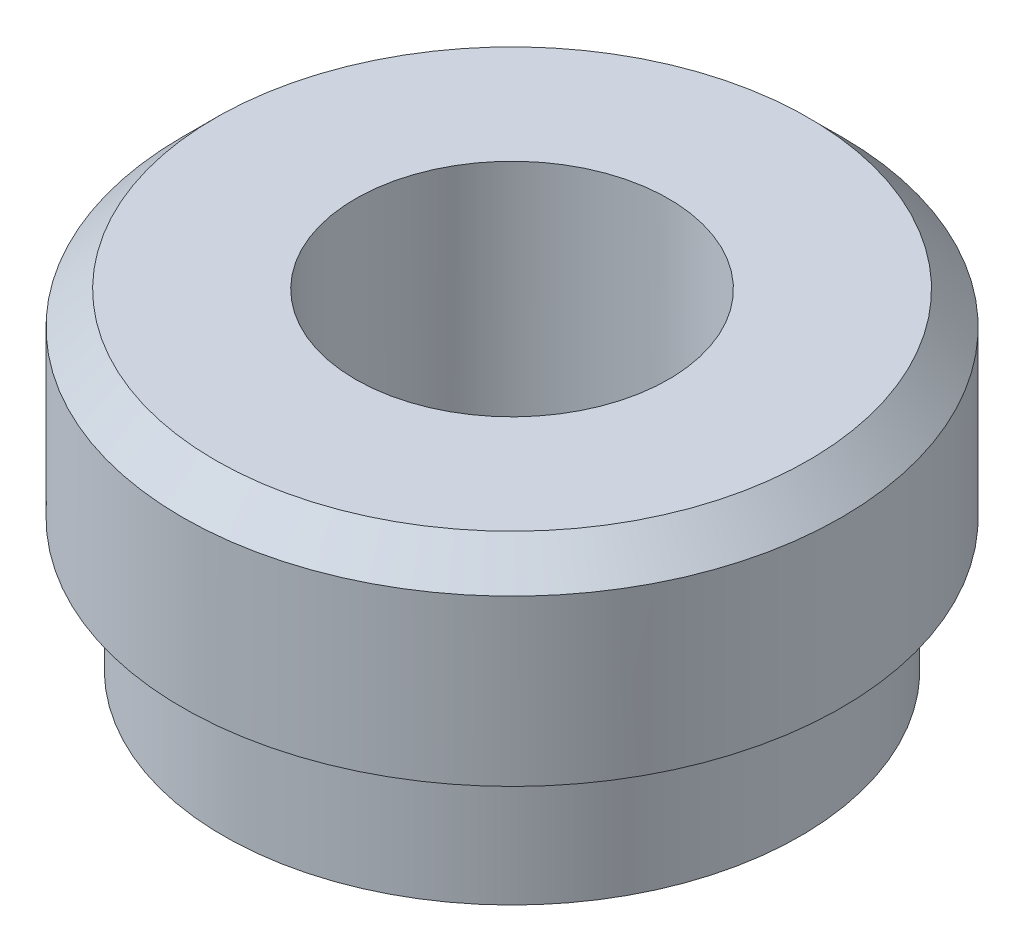
SolidWorks part; units mm, degrees
material "Q235"
ref_plane "Front Plane" through (0, 0, 0) normal (0, 0, 1) x (1, 0, 0)
ref_plane "Top Plane" through (0, 0, 0) normal (0, 1, 0) x (1, 0, 0)
ref_plane "Right Plane" through (0, 0, 0) normal (1, 0, 0) x (0, 0, -1)
sketch "Sketch1" plane through (0, 0, 0) normal (0, 0, 1) x (1, 0, 0)
  line L0 (0, 0) -> (20, 0)
  line L1 (20, 0) -> (20, -12)
  line L2 (20, -12) -> (17.5, -12)
  line L3 (17.5, -12) -> (17.5, -20)
  line L4 (17.5, -20) -> (0, -20)
  line L5 (0, -20) -> (0, 0)
  dimension "D1" = 17.5
  dimension "D2" = 20
  dimension "D3" = 8
  dimension "D4" = 12
revolve "Revolve1" add sketch "Sketch1" angle 360 about L5
hole_wizard "G1/2 Tapped Hole1" positions "Sketch2" profile "Sketch3" tap size "G1/2" standard "GB"
sketch "Sketch2" plane through (0, 0, 0) normal (0, 1, 0) x (1, 0, 0)
  point P0 (0, 0)
sketch "Sketch3" plane through (0, 0, 0) normal (1, 0, 0) x (0, 0, 1)
  line L0 (0, 0) -> (0, 53.0582)
  line L1 (0, 53.0582) -> (9.5, 47.35)
  line L2 (9.5, 47.35) -> (9.5, 0)
  line L5 (9.5, 0) -> (0, 0)
  line L10 (0, 53.0582) -> (-9.5, 47.35) construction
  line L11 (0, -6.35) -> (0, 107.95) construction
  dimension "螺纹孔钻头直径" = 19
  dimension "螺纹孔钻头深度" = 47.35
  dimension "导头角度" = 118
cosmetic thread "Hole cosmetic thread1" parameters "D1"=20, "D2"=20.955
chamfer "Chamfer1" distance 2 angle 45 1 edges at (0, 0, -20)
